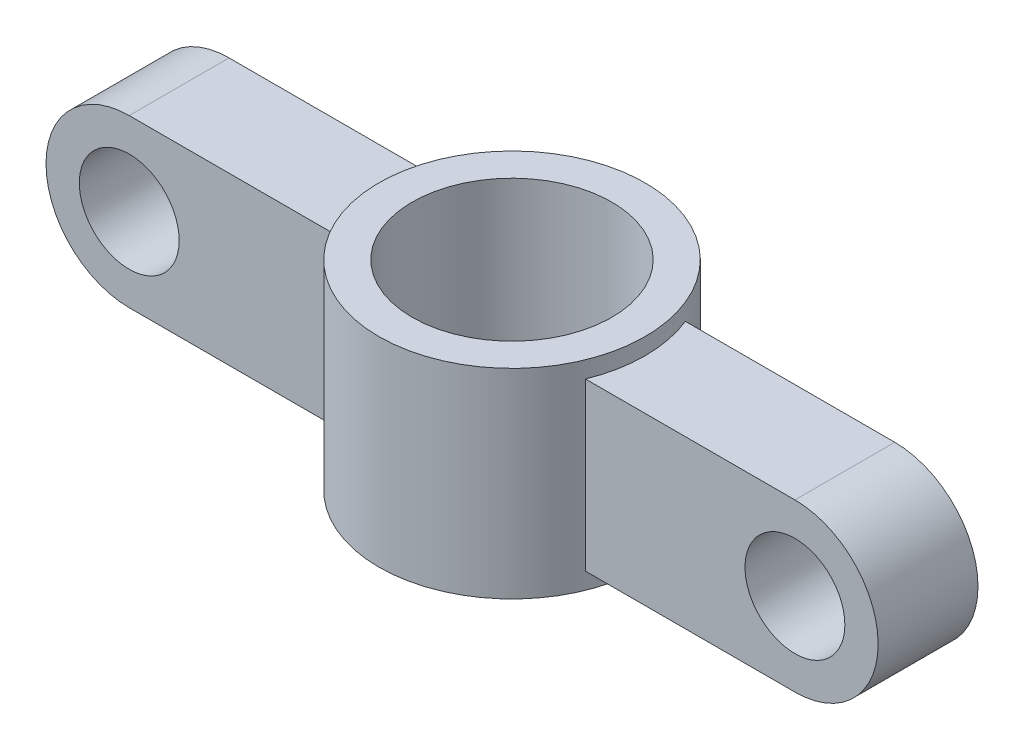
from build123d import *

# Parameters (mm, degrees)
SKETCH1_R           = 4
SKETCH1_R_2         = 3
BOSS_EXTRUDE1_DEPTH = 6
SKETCH2_R           = 2.5
SKETCH2_R_2         = 1.5
BOSS_EXTRUDE2_DEPTH = 1.5


with BuildPart() as part:
    # Sketch1 → Boss-Extrude1 (new body)
    with BuildSketch(Plane(origin=(0, 0, 0), x_dir=(1, 0, 0), z_dir=(0, 1, 0))):
        with Locations(Location((0, 0, 0), (0, 0, 270))):
            Circle(SKETCH1_R)
        with Locations(Location((0, 0, 0), (0, 0, 270))):
            Circle(SKETCH1_R_2, mode=Mode.SUBTRACT)
    extrude(amount=BOSS_EXTRUDE1_DEPTH)

    # Sketch2 → Boss-Extrude2 (add, symmetric)
    # profile 1 of 4: a face of its own
    with BuildSketch(Plane.XY):
        with BuildLine():
            Line((-3, 5.5), (-10, 5.5))
            ThreePointArc((-10, 5.5), (-8.232233047, 4.767766953), (-7.5, 3))
            ThreePointArc((-7.5, 3), (-8.232233047, 1.232233047), (-10, 0.5))
            Line((-10, 0.5), (-3, 0.5))
            Line((-3, 0.5), (-3, 5.5))
        make_face()
    # profile 2 of 4: a face of its own
    with BuildSketch(Plane.XY):
        with Locations((-10, 3)):
            Circle(SKETCH2_R)
        with Locations((-10, 3)):
            Circle(SKETCH2_R_2, mode=Mode.SUBTRACT)
    # profile 3 of 4: a face of its own
    with BuildSketch(Plane.XY):
        with BuildLine():
            Line((3, 5.5), (3, 0.5))
            Line((3, 0.5), (10, 0.5))
            ThreePointArc((10, 0.5), (7.5, 3), (10, 5.5))
            Line((10, 5.5), (3, 5.5))
        make_face()
    # profile 4 of 4: a face of its own
    with BuildSketch(Plane.XY):
        with Locations((10, 3)):
            Circle(SKETCH2_R)
        with Locations((10, 3)):
            Circle(SKETCH2_R_2, mode=Mode.SUBTRACT)
    extrude(amount=BOSS_EXTRUDE2_DEPTH, both=True)


solid = part.part
